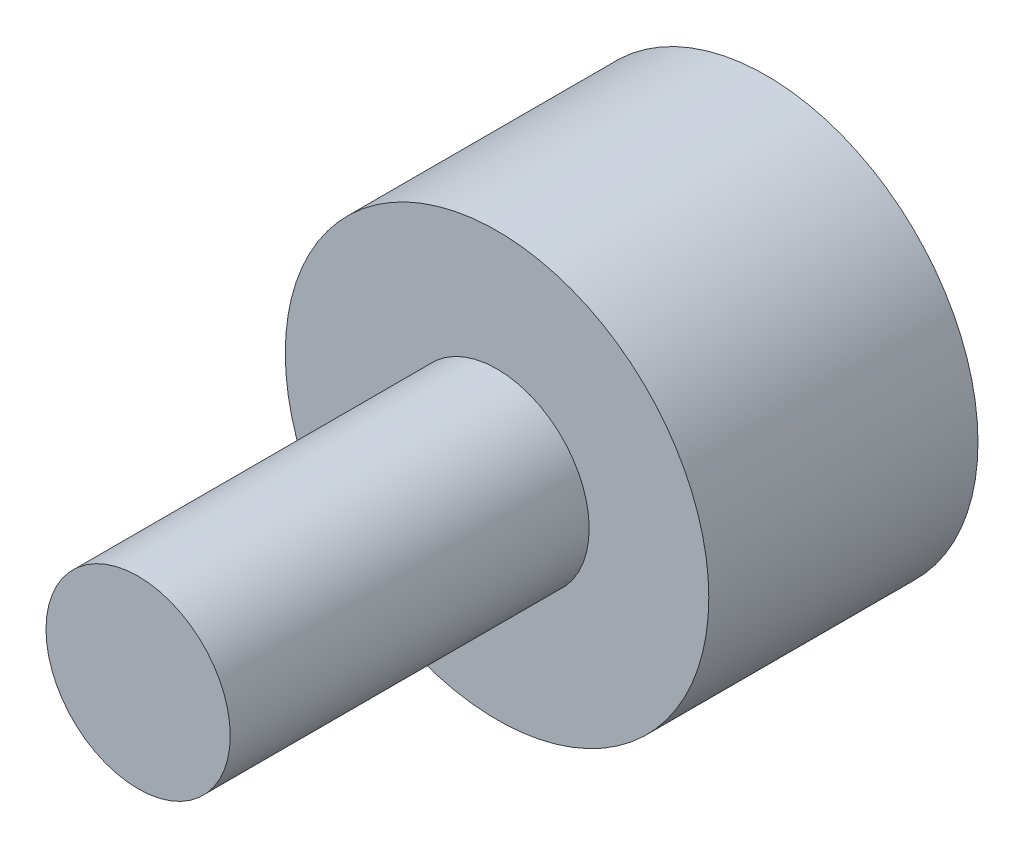
SolidWorks part; units mm, degrees
material "1060 合金"
ref_plane "前视基准面" through (0, 0, 0) normal (0, 0, 1) x (1, 0, 0)
ref_plane "上视基准面" through (0, 0, 0) normal (0, 1, 0) x (1, 0, 0)
ref_plane "右视基准面" through (0, 0, 0) normal (1, 0, 0) x (0, 0, -1)
other "Configuration Table"
sketch "草图1" plane through (0, 0, 0) normal (0, 0, 1) x (1, 0, 0)
  circle A0 centre (0, 0) radius 3.54
  dimension "D1" = 7.08
extrude "凸台-拉伸1" add sketch "草图1" along normal blind 4.5 contours A0
sketch "草图2" plane through (0, 0, 4.5) normal (0, 0, 1) x (1, 0, 0)
  circle A0 centre (0, 0) radius 1.54
  dimension "D1" = 3.08
extrude "凸台-拉伸2" add sketch "草图2" along normal blind 6
